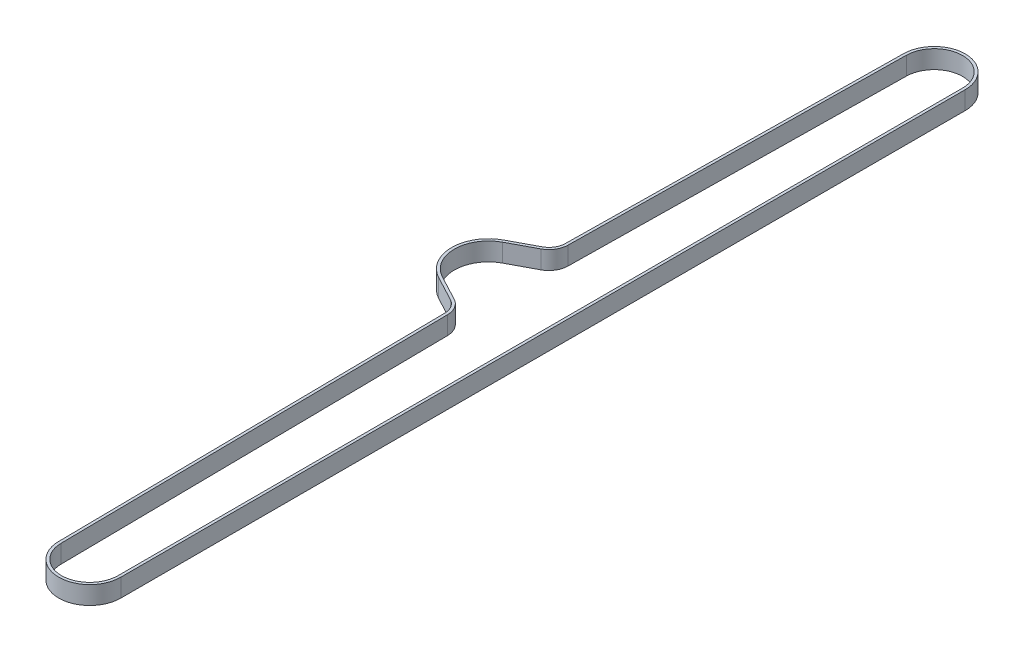
from build123d import *

# Parameters (mm, degrees)
EXTRUDE_1_DEPTH = 15


with BuildPart() as part:
    # 草图1 → 拉伸-薄壁1 (new, symmetric)
    with BuildSketch(Plane(origin=(-54.389817032, 234.459616021, 1948), x_dir=(0, 0, 1), z_dir=(0, -1, 0))):
        with BuildLine():
            Line((-669.781125, 73.589656521), (-691.82105475, 115.041248428))
            ThreePointArc((-691.82105475, 115.041248428), (-745.5, 147.295), (-799.17894525, 115.041248428))
            Line((-799.17894525, 115.041248428), (-821.218875, 73.589656521))
            ThreePointArc((-821.218875, 73.589656521), (-831.170890239, 63.02817405), (-845.113030011, 59.002722785))
            Line((-845.113030011, 59.002722785), (-1396.721100985, 51.239926214))
            ThreePointArc((-1396.721100985, 51.239926214), (-1447.243731538, -0.360559418), (-1396, -51.245))
            Line((-1396, -51.245), (0, -51.245))
            ThreePointArc((0, -51.245), (51.244076889, -0.307585387), (0.615159693, 51.24130759))
            Line((0.615159693, 51.24130759), (-645.830117895, 59.001981486))
            ThreePointArc((-645.830117895, 59.001981486), (-659.804837816, 63.013373698), (-669.781125, 73.589656521))
        make_face()
        with BuildLine():
            Line((-673.7544, 71.477054861), (-695.79432975, 112.928646768))
            ThreePointArc((-695.79432975, 112.928646768), (-745.5, 142.795), (-795.20567025, 112.928646768))
            Line((-795.20567025, 112.928646768), (-817.2456, 71.477054861))
            ThreePointArc((-817.2456, 71.477054861), (-828.826126823, 59.187329803), (-845.049707649, 54.503168332))
            Line((-845.049707649, 54.503168332), (-1396.657778624, 46.74037176))
            ThreePointArc((-1396.657778624, 46.74037176), (-1442.743842926, -0.328897453), (-1396, -46.745))
            Line((-1396, -46.745), (0, -46.745))
            ThreePointArc((0, -46.745), (46.744157951, -0.280575254), (0.561140401, 46.741631833))
            Line((0.561140401, 46.741631833), (-645.884137187, 54.50230573))
            ThreePointArc((-645.884137187, 54.50230573), (-662.145629459, 59.170107576), (-673.7544, 71.477054861))
        make_face(mode=Mode.SUBTRACT)
    extrude(amount=EXTRUDE_1_DEPTH, both=True)


solid = part.part
